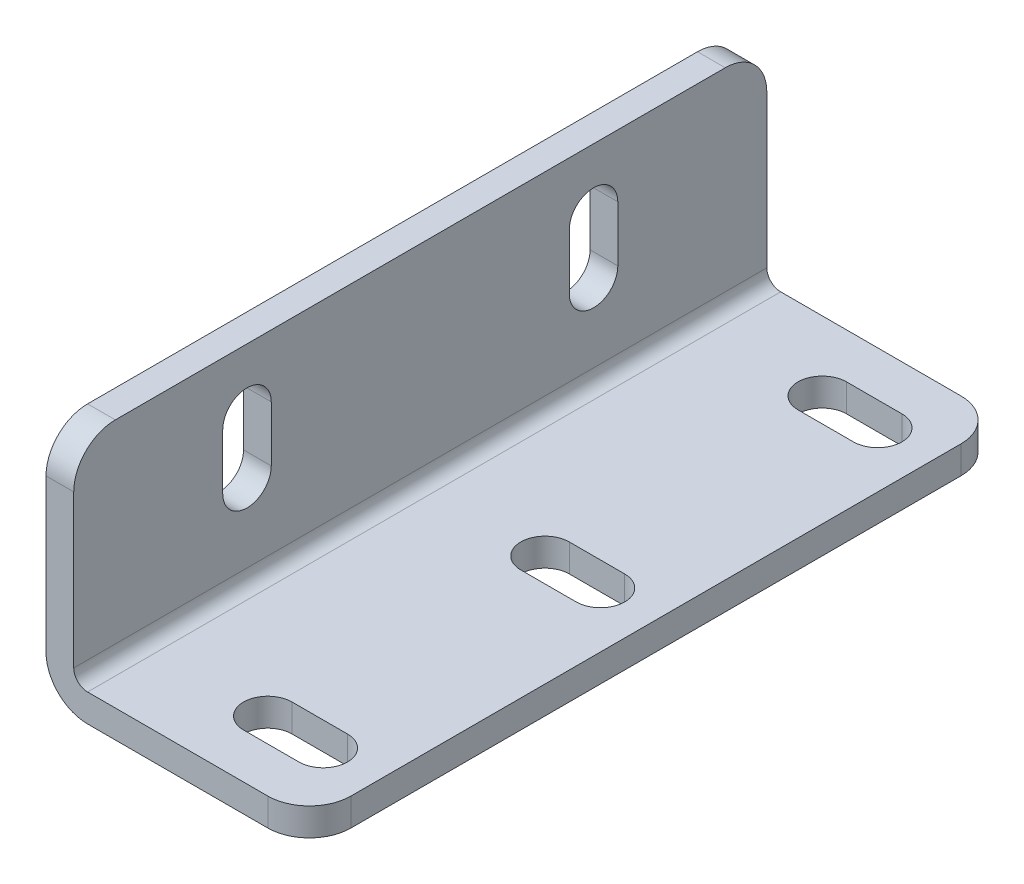
SolidWorks part; units mm, degrees
material "6061 合金"
ref_plane "前视基准面" through (0, 0, 0) normal (0, 0, 1) x (1, 0, 0)
ref_plane "上视基准面" through (0, 0, 0) normal (0, 1, 0) x (1, 0, 0)
ref_plane "右视基准面" through (0, 0, 0) normal (1, 0, 0) x (0, 0, -1)
sketch "草图9" plane through (0, 0, 0) normal (0, 0, 1) x (1, 0, 0)
  line L0 (0, 0) -> (0, 15)
  line L1 (0, 0) -> (17, 0)
  dimension "D1" = 17
  dimension "D2" = 15
extrude "拉伸-薄壁1" add sketch "草图9" along normal mid plane 50 thin thin type one direction wall 2
sketch "草图10" plane through (0, 0, 0) normal (0, 1, 0) x (1, 0, 0)
  line L0 (-9.4418, 20) -> (20.3442, 20) construction
  line L1 (9, 20) -> (13, 20) construction
  line L2 (9, 21.75) -> (13, 21.75)
  line L3 (9, 18.25) -> (13, 18.25)
  line L4 (0, 0) -> (41.5624, 0) construction
  line L5 (9, -20) -> (13, -20) construction
  line L6 (9, -21.75) -> (13, -21.75)
  line L7 (9, -18.25) -> (13, -18.25)
  line L8 (17, -25) -> (17, 25) construction
  line L9 (9, 0) -> (13, 0) construction
  line L10 (9, 1.75) -> (13, 1.75)
  line L11 (9, -1.75) -> (13, -1.75)
  arc A0 (9, 21.75) -> (9, 18.25) centre (9, 20) ccw
  arc A1 (13, 18.25) -> (13, 21.75) centre (13, 20) ccw
  arc A2 (9, -21.75) -> (9, -18.25) centre (9, -20) cw
  arc A3 (13, -18.25) -> (13, -21.75) centre (13, -20) cw
  arc A4 (9, 1.75) -> (9, -1.75) centre (9, 0) ccw
  arc A5 (13, -1.75) -> (13, 1.75) centre (13, 0) ccw
  point P4 (11, 20)
  point P14 (11, -20)
  point P23 (11, 0)
  dimension "D4" = 1.75
  dimension "D1" = 4
  dimension "D2" = 6
  dimension "D3" = 20
  dimension "D5" = 1.75
  dimension "D6" = 4
  dimension "D7" = 6
extrude "切除-拉伸1" cut sketch "草图10" against normal blind 10
sketch "草图11" plane through (0, 0, 0) normal (1, 0, 0) x (0, 0, -1)
  line L0 (-12.5, 10.5) -> (-12.5, 6.5) construction
  line L1 (-10.75, 10.5) -> (-10.75, 6.5)
  line L2 (-14.25, 10.5) -> (-14.25, 6.5)
  line L3 (-25, 15) -> (25, 15) construction
  line L4 (0, 0) -> (0, 40.1643) construction
  line L5 (12.5, 10.5) -> (12.5, 6.5) construction
  line L6 (10.75, 10.5) -> (10.75, 6.5)
  line L7 (14.25, 10.5) -> (14.25, 6.5)
  arc A0 (-10.75, 10.5) -> (-14.25, 10.5) centre (-12.5, 10.5) ccw
  arc A1 (-14.25, 6.5) -> (-10.75, 6.5) centre (-12.5, 6.5) ccw
  arc A2 (10.75, 10.5) -> (14.25, 10.5) centre (12.5, 10.5) cw
  arc A3 (14.25, 6.5) -> (10.75, 6.5) centre (12.5, 6.5) cw
  point P2 (-12.5, 8.5)
  point P14 (12.5, 8.5)
  dimension "D1" = 1.75
  dimension "D2" = 4
  dimension "D3" = 6.5
  dimension "D4" = 25
extrude "切除-拉伸2" cut sketch "草图11" against normal blind 10
fillet "圆角1" radius 3 4 edges at (-1, 15, 25) (-1, 15, -25) (17, -1, 25) (17, -1, -25)
fillet "圆角2" radius 1 1 edges at (0, 0, 0)
fillet "圆角3" radius 3 1 edges at (-2, -2, 0)
